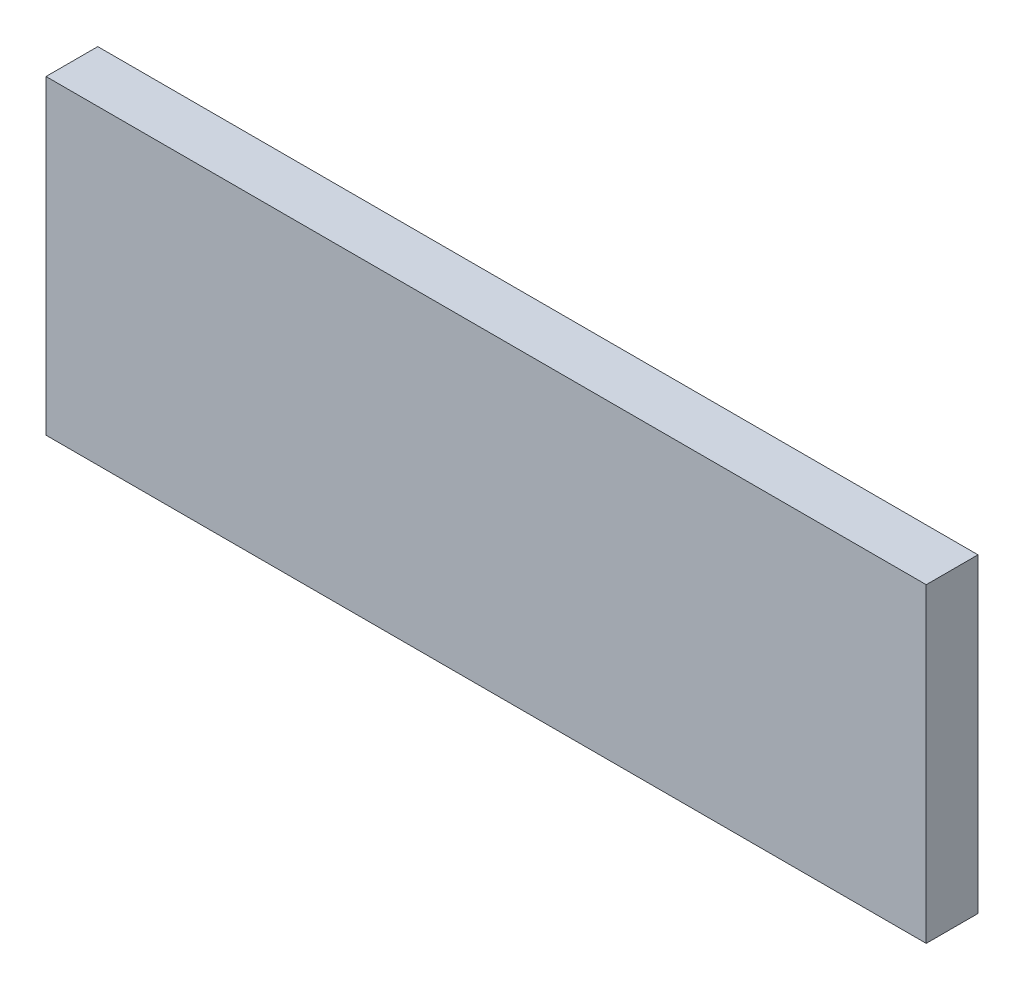
from build123d import *

# Parameters (mm, degrees)
SKETCH1_W           = 340
SKETCH1_H           = 120
BOSS_EXTRUDE1_DEPTH = 20


with BuildPart() as part:
    # Sketch1 → Boss-Extrude1 (new body)
    with BuildSketch(Plane.XY):
        with Locations((170, 60)):
            Rectangle(SKETCH1_W, SKETCH1_H)
    extrude(amount=BOSS_EXTRUDE1_DEPTH)


solid = part.part
